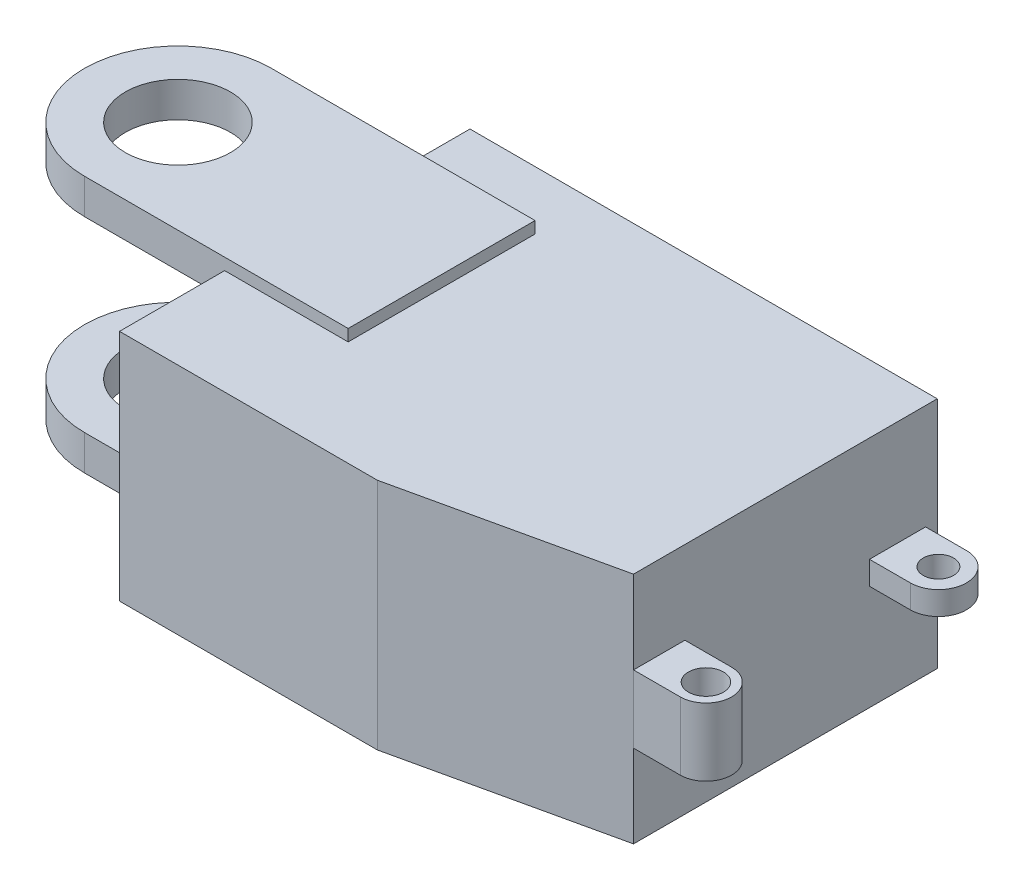
from build123d import *

# Parameters (mm, degrees)
SKETCH1_W                = 400
SKETCH1_H                = 300
BOSS_EXTRUDE1_DEPTH      = 200
BOSS_EXTRUDE2_DEPTH      = 29
BOSS_EXTRUDE2_DEPTH_BACK = 29
SKETCH2_R                = 15
CUT_EXTRUDE1_DEPTH       = 363.138095207
BOSS_EXTRUDE3_START      = -20
SKETCH4_R                = 45
BOSS_EXTRUDE3_DEPTH      = 30
BOSS_EXTRUDE4_DEPTH      = 10
BOSS_EXTRUDE4_DEPTH_BACK = 10
SKETCH5_R                = 13


with BuildPart() as part:
    # Sketch1 → Boss-Extrude1 (new body)
    with BuildSketch(Plane(origin=(0, 0, 0), x_dir=(1, 0, 0), z_dir=(0, 1, 0))):
        Rectangle(SKETCH1_W, SKETCH1_H)
    extrude(amount=BOSS_EXTRUDE1_DEPTH)

    # Sketch2 → Boss-Extrude2 (add, two sides: drawn at the far end of the back side and taken through both)
    with BuildSketch(Plane(origin=(0, 100, 0), x_dir=(1, 0, 0), z_dir=(0, 1, 0)).offset(-BOSS_EXTRUDE2_DEPTH_BACK)):
        with BuildLine():
            Line((187.36144438, -66), (240, -66))
            ThreePointArc((240, -66), (262, -88), (240, -110))
            Line((240, -110), (187.36144438, -110))
            Line((187.36144438, -110), (187.36144438, -66))
        make_face()
        with Locations(Location((240, -88, 0), (0, 0, 270))):
            Circle(SKETCH2_R, mode=Mode.SUBTRACT)
    extrude(amount=BOSS_EXTRUDE2_DEPTH + BOSS_EXTRUDE2_DEPTH_BACK)

    # Sketch3 → Cut-Extrude1 (cut, through all)
    with BuildSketch(Plane(origin=(0, 200, 0), x_dir=(1, 0, 0), z_dir=(0, 1, 0))):
        Polygon((200, -110), (20.728700198, -150), (200, -150), align=None)
    extrude(amount=-CUT_EXTRUDE1_DEPTH, mode=Mode.SUBTRACT)

    # Sketch4 → Boss-Extrude3 (add)
    with BuildSketch(Plane(origin=(0, 200, 0), x_dir=(1, 0, 0), z_dir=(0, 1, 0)).offset(BOSS_EXTRUDE3_START)):
        with BuildLine():
            Line((-94.278565111, -60), (-320, -60))
            ThreePointArc((-320, -60), (-400, 20), (-320, 100))
            Line((-320, 100), (-94.278565111, 100))
            Line((-94.278565111, 100), (-94.278565111, -60))
        make_face()
        with Locations(Location((-320, 20, 0), (0, 0, 270))):
            Circle(SKETCH4_R, mode=Mode.SUBTRACT)
    boss_extrude3 = extrude(amount=BOSS_EXTRUDE3_DEPTH)

    # Mirror1: Boss-Extrude3 across plane
    add(boss_extrude3.mirror(Plane.ZX.offset(100)))

    # Sketch5 → Boss-Extrude4 (add, two sides: drawn at the far end of the back side and taken through both)
    with BuildSketch(Plane(origin=(0, 100, 0), x_dir=(1, 0, 0), z_dir=(0, 1, 0)).offset(-BOSS_EXTRUDE4_DEPTH_BACK)):
        with BuildLine():
            Line((184.247820943, 140), (235, 140))
            ThreePointArc((235, 140), (259, 116), (235, 92))
            Line((235, 92), (184.247820943, 92))
            Line((184.247820943, 92), (184.247820943, 140))
        make_face()
        with Locations(Location((235, 116, 0), (0, 0, 270))):
            Circle(SKETCH5_R, mode=Mode.SUBTRACT)
    extrude(amount=BOSS_EXTRUDE4_DEPTH + BOSS_EXTRUDE4_DEPTH_BACK)


solid = part.part
